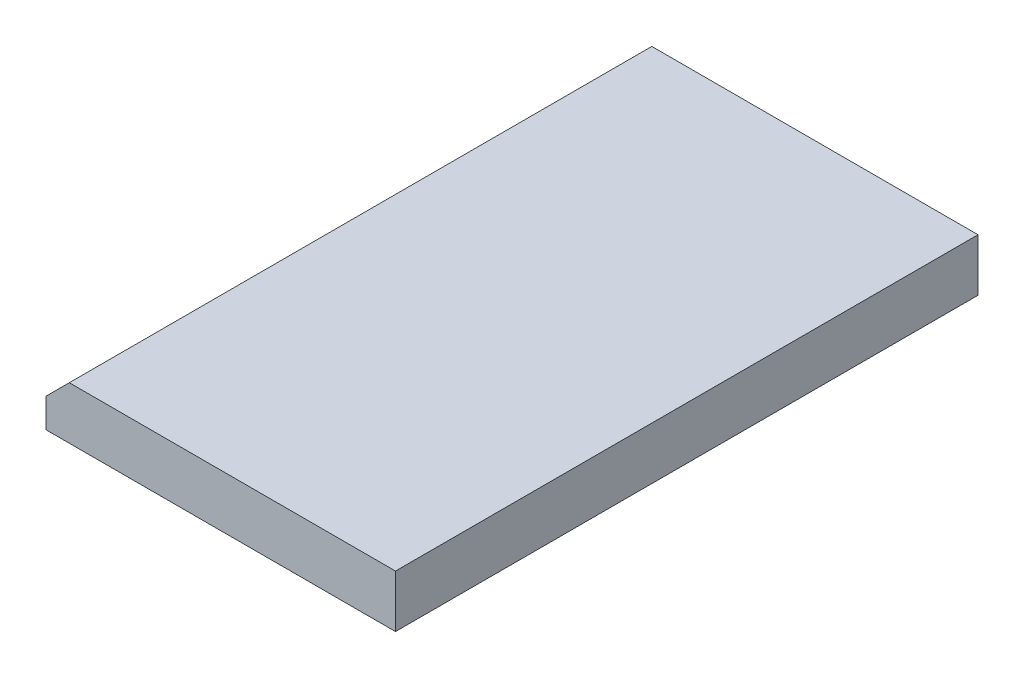
SolidWorks part; units mm, degrees
ref_plane "Front Plane" through (0, 0, 0) normal (0, 0, 1) x (1, 0, 0)
ref_plane "Top Plane" through (0, 0, 0) normal (0, 1, 0) x (1, 0, 0)
ref_plane "Right Plane" through (0, 0, 0) normal (1, 0, 0) x (0, 0, -1)
other "Configuration Table"
sketch "Sketch1" plane through (0, 0, 0) normal (0, 1, 0) x (1, 0, 0)
  line L1 (-6, -10) -> (6, -10)
  line L2 (-6, -10) -> (-6, 10)
  line L3 (-6, 10) -> (6, 10)
  line L4 (6, -10) -> (6, 10)
  line L5 (-6, -10) -> (6, 10) construction
  line L6 (-6, 10) -> (6, -10) construction
  point P0 (0, 0)
  dimension "D1" = 20
  dimension "D2" = 12
extrude "Boss-Extrude2" add sketch "Sketch1" along normal blind 1.8
sketch "Sketch2" plane through (0, 0, 0) normal (0, 0, 1) x (1, 0, 0)
  line L0 (-6, 1) -> (-5.2, 1.8)
  line L1 (-6, 1.8) -> (-6, 0) construction
  line L2 (-6, 1.8) -> (6, 1.8) construction
  line L3 (-5.2, 1.8) -> (-6, 1.8)
  line L4 (-6, 1.8) -> (-6, 1)
  line L5 (-6, 0) -> (6, 0) construction
  dimension "D1" = 1
  dimension "D2" = 45
extrude "Cut-Extrude1" cut sketch "Sketch2" against normal through all both and the other way through all
